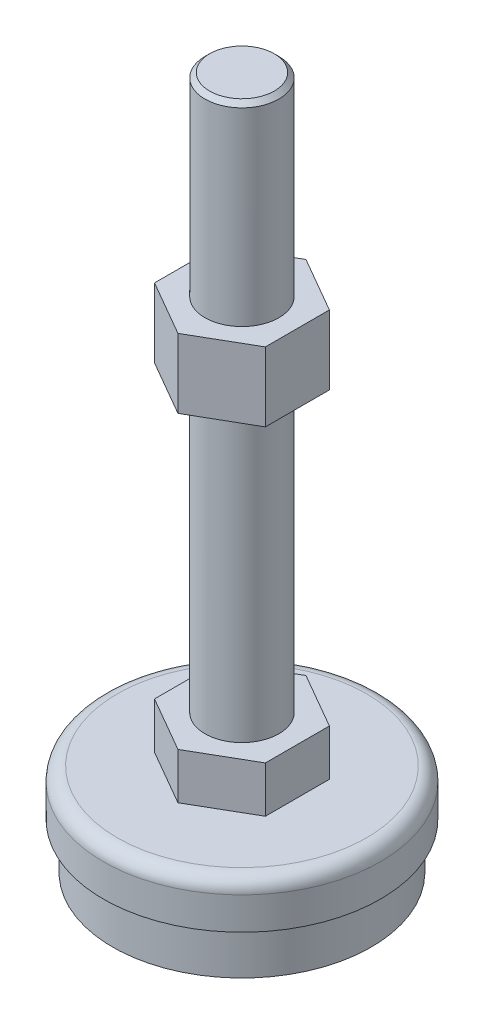
from build123d import *

# Parameters (mm, degrees)
SKETCH_2_R      = 8
EXTRUDE_1_DEPTH = 10
EXTRUDE_START   = 63
EXTRUDE_2_DEPTH = 15
CHAMFER_1_SIZE  = 1


with BuildPart() as part:
    # 草图1 → 旋转1 (revolve)
    with BuildSketch(Plane.XY, mode=Mode.PRIVATE) as revolve_1_sk:
        with BuildLine():
            Line((0, 0), (0, 150))
            Line((0, 150), (8, 150))
            Line((8, 150), (8, 20))
            Line((8, 20), (27, 20))
            ThreePointArc((27, 20), (29.121320344, 19.121320344), (30, 17))
            Line((30, 17), (30, 10))
            Line((30, 10), (28, 10))
            Line((28, 10), (28, 0))
            Line((28, 0), (0, 0))
        make_face()
    revolve(revolve_1_sk.sketch.rotate(Axis((0, 0, 0), (0, 1, 0)), 90), axis=Axis((0, 0, 0), (0, 1, 0)))

    # 倒角1
    chamfer_1_edges = [part.edges().sort_by_distance(p)[0] for p in [
        (0, 150, 8),
    ]]
    chamfer(chamfer_1_edges, length=CHAMFER_1_SIZE)


with BuildPart() as body_2:
    # 草图2 → 凸台-拉伸1 (new body)
    with BuildSketch(Plane(origin=(0, 20, 0), x_dir=(1, 0, 0), z_dir=(0, 1, 0))):
        Polygon((0, 13.856406461), (-12, 6.92820323), (-12, -6.92820323), (0, -13.856406461), (12, -6.92820323), (12, 6.92820323), align=None)
        with Locations(Location((0, 0, 0), (0, 0, 270))):
            Circle(SKETCH_2_R, mode=Mode.SUBTRACT)
    extrude(amount=EXTRUDE_1_DEPTH)


with BuildPart() as body_3:
    # 草图4 → 凸台-拉伸2 (new body)
    with BuildSketch(Plane(origin=(0, 30, 0), x_dir=(1, 0, 0), z_dir=(0, 1, 0)).offset(EXTRUDE_START)):
        Polygon((12, 6.92820323), (0, 13.856406461), (-12, 6.92820323), (-12, -6.92820323), (0, -13.856406461), (12, -6.92820323), align=None)
    extrude(amount=EXTRUDE_2_DEPTH)


solid = Compound([part.part, body_2.part, body_3.part])
